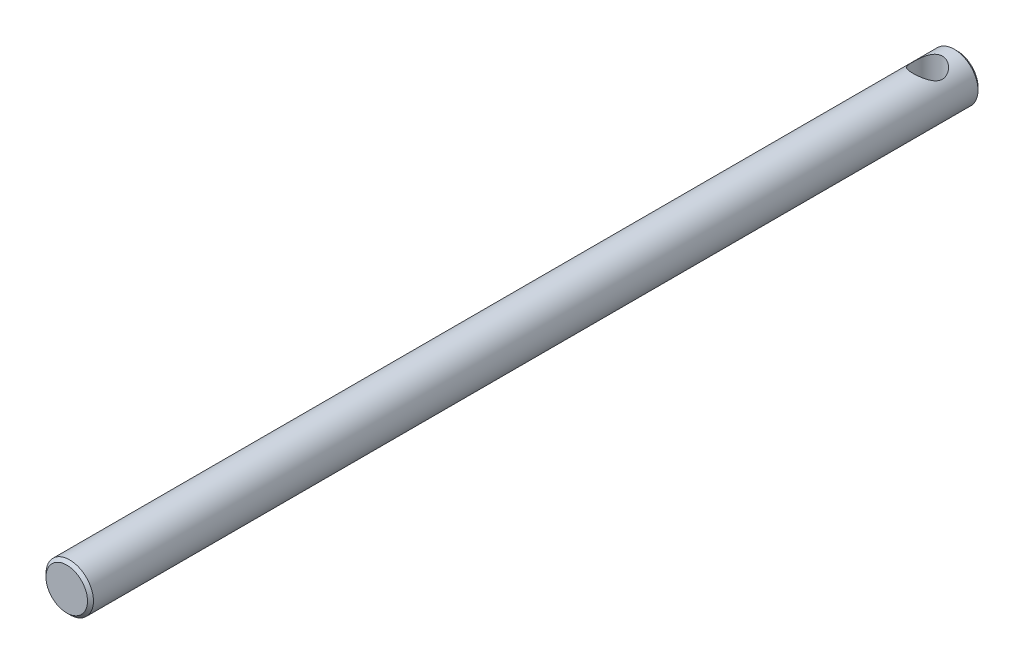
SolidWorks part; units mm, degrees
ref_plane "Front Plane" through (0, 0, 0) normal (0, 0, 1) x (1, 0, 0)
ref_plane "Top Plane" through (0, 0, 0) normal (0, 1, 0) x (1, 0, 0)
ref_plane "Right Plane" through (0, 0, 0) normal (1, 0, 0) x (0, 0, -1)
sketch "Sketch1" plane through (0, 0, 0) normal (0, 0, 1) x (1, 0, 0)
  circle A0 centre (0, 0) radius 4
  dimension "D1" = 8
extrude "Boss-Extrude1" add sketch "Sketch1" along normal mid plane 150
sketch "Sketch2" plane through (0, 0, 0) normal (0, 1, 0) x (1, 0, 0)
  circle A0 centre (0, 70) radius 2.5
  dimension "D1" = 5
  dimension "D2" = 70
extrude "Cut-Extrude1" cut sketch "Sketch2" against normal mid plane 150
chamfer "Chamfer1" distance 0.5 angle 45 2 edges at (4, 0, 75) (4, 0, -75)
